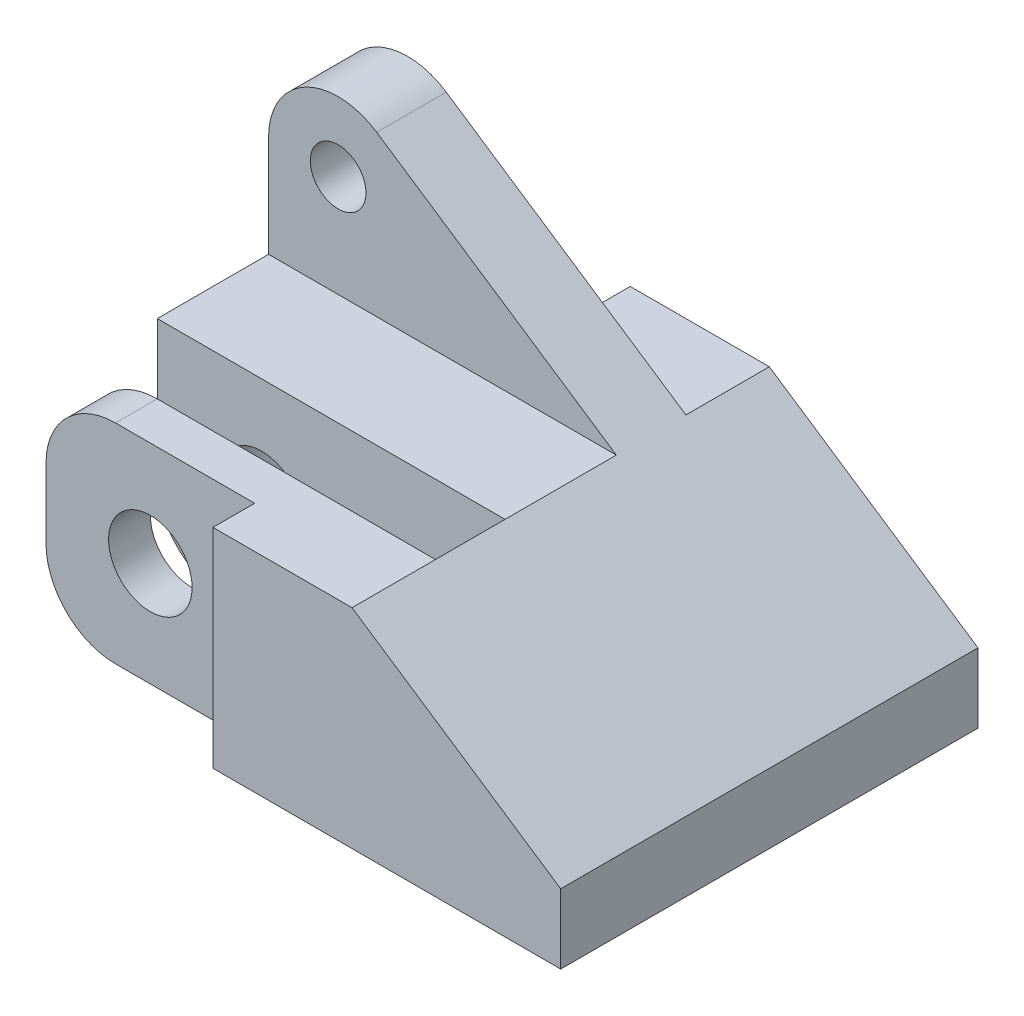
SolidWorks part; units mm, degrees
ref_plane "Front Plane" through (0, 0, 0) normal (0, 0, 1) x (1, 0, 0)
ref_plane "Top Plane" through (0, 0, 0) normal (0, 1, 0) x (1, 0, 0)
ref_plane "Right Plane" through (0, 0, 0) normal (1, 0, 0) x (0, 0, -1)
other "Configuration Table"
sketch "Sketch1" plane through (0, 0, 0) normal (0, 0, 1) x (1, 0, 0)
  line L0 (0, 0) -> (0, 5)
  line L1 (0, 5) -> (-15, 15)
  line L2 (-15, 15) -> (-40, 15)
  line L3 (-40, 15) -> (-40, 0)
  line L4 (-40, 0) -> (0, 0)
  dimension "D1" = 40
  dimension "D2" = 25
  dimension "D3" = 5
  dimension "D4" = 15
extrude "Boss-Extrude1" add sketch "Sketch1" along normal mid plane 30
sketch "Sketch2" plane through (0, 15, 0) normal (0, 1, 0) x (1, 0, 0)
  line L0 (0, 0) -> (-48.8783, 0) construction
  line L1 (-40, -15) -> (-40, 15) construction
  line L2 (-63.1994, 32.3578) -> (-25, 32.3578)
  line L3 (-63.1994, 32.3578) -> (-63.1994, 12)
  line L4 (-63.1994, 12) -> (-25, 12)
  line L5 (-25, 32.3578) -> (-25, 12)
  line L6 (-44.0997, 12) -> (-44.0997, 32.3578) construction
  line L7 (-63.1994, 22.1789) -> (-25, 22.1789) construction
  line L8 (-63.1994, -22.1789) -> (-25, -22.1789) construction
  line L9 (-44.0997, -12) -> (-44.0997, -32.3578) construction
  line L10 (-25, -32.3578) -> (-25, -12)
  line L11 (-63.1994, -12) -> (-25, -12)
  line L12 (-63.1994, -32.3578) -> (-63.1994, -12)
  line L13 (-63.1994, -32.3578) -> (-25, -32.3578)
  point P3 (-44.0997, 22.1789)
  point P17 (-44.0997, -22.1789)
  dimension "D1" = 15
  dimension "D2" = 24
extrude "Cut-Extrude1" cut sketch "Sketch2" against normal blind 30
sketch "Sketch3" plane through (0, 15, 0) normal (0, 1, 0) x (1, 0, 0)
  line L0 (-40, -12) -> (-40, 12) construction
  line L1 (-40, -4) -> (-15, -4)
  line L2 (-40, -4) -> (-40, -9)
  line L3 (-40, -9) -> (-15, -9)
  line L4 (-15, -4) -> (-15, -9)
  line L5 (-15, -15) -> (-15, 15) construction
  line L6 (-15, -15) -> (-25, -15) construction
  dimension "D1" = 5
  dimension "D2" = 6
extrude "Cut-Extrude2" cut sketch "Sketch3" against normal blind 30
sketch "Sketch4" plane through (0, 0, -15) normal (0, 0, 1) x (1, 0, 0)
  line L0 (-15, 15) -> (-32.2265, 26.4843)
  line L1 (0, 5) -> (-15, 15) construction
  line L2 (-40, 15) -> (-40, 22.3241)
  line L3 (-40, 15) -> (-15, 15)
  arc A0 (-32.2265, 26.4843) -> (-40, 22.3241) centre (-35, 22.3241) ccw
  circle A1 centre (-35, 22.3241) radius 2
  dimension "D1" = 5
  dimension "D2" = 4
extrude "Boss-Extrude3" add sketch "Sketch4" along normal blind 5 from offset 6
sketch "Sketch5" plane through (0, 0, 12) normal (0, 0, 1) x (1, 0, 0)
  line L0 (-40, 0) -> (-40, 15) construction
  line L1 (-25, 0) -> (-40, 0) construction
  circle A0 centre (-32.5, 7.5) radius 3
  dimension "D1" = 6
  dimension "D2" = 7.5
  dimension "D3" = 7.5
extrude "Cut-Extrude3" cut sketch "Sketch5" against normal blind 27
fillet "Fillet1" radius 5 2 edges at (-40, 15, 10.5) (-40, 0, 10.5)
fillet "Fillet2" radius 5 1 edges at (-40, 0, -4)
